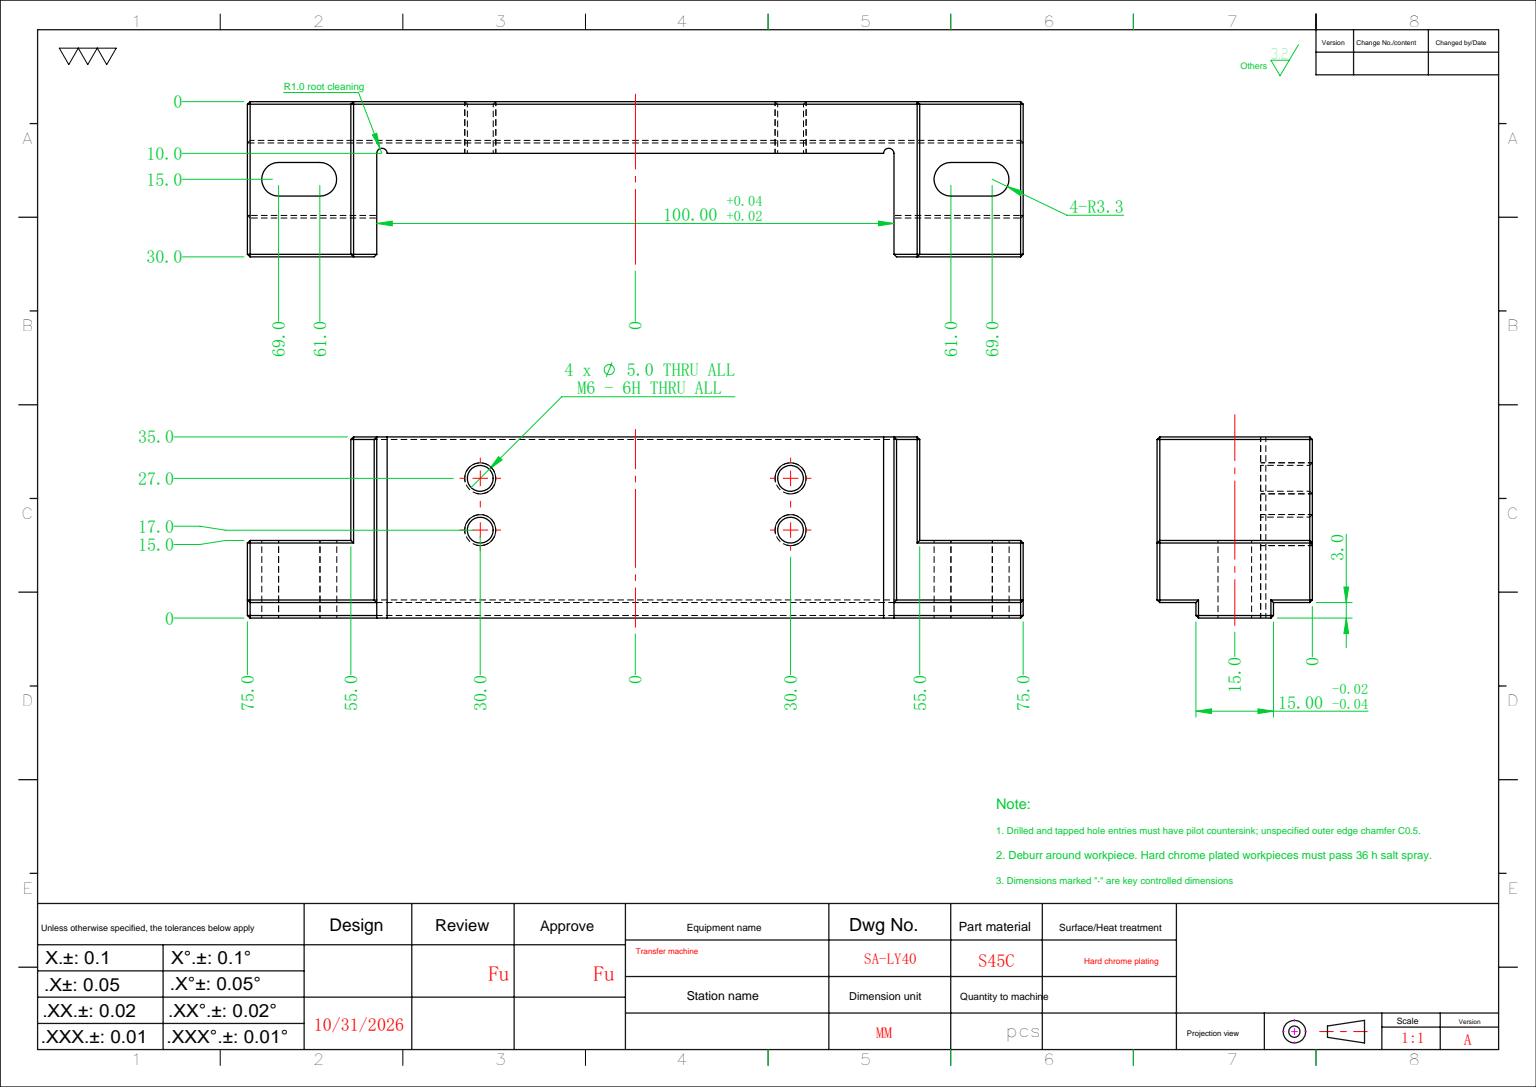
SolidWorks part; units mm, degrees
material "S45C"
ref_plane "前视基准面" through (0, 0, 0) normal (0, 0, 1) x (1, 0, 0)
ref_plane "上视基准面" through (0, 0, 0) normal (0, 1, 0) x (1, 0, 0)
ref_plane "右视基准面" through (0, 0, 0) normal (1, 0, 0) x (0, 0, -1)
sketch "草图1" plane through (0, 0, 0) normal (0, 0, 1) x (1, 0, 0)
  line L0 (0, 0) -> (116.7587, 0) construction
  line L1 (0, 0) -> (0, 69.0405) construction
  line L2 (-75, 0) -> (-75, 15)
  line L3 (-75, 15) -> (-55, 15)
  line L4 (-55, 15) -> (-55, 35)
  line L5 (55, 15) -> (55, 35)
  line L6 (75, 15) -> (55, 15)
  line L7 (75, 0) -> (75, 15)
  line L8 (-75, 0) -> (75, 0)
  line L9 (-55, 35) -> (55, 35)
  dimension "D1" = 150
  dimension "D2" = 110
  dimension "D3" = 15
  dimension "D4" = 35
extrude "凸台-拉伸1" add sketch "草图1" along normal mid plane 30
sketch "草图2" plane through (-75, 0, 0) normal (-1, 0, 0) x (0, 0, 1)
  line L0 (0, 0) -> (0, 17.2771) construction
  line L1 (-15, 0) -> (-7.5, 0)
  line L2 (-15, 0) -> (-15, 3)
  line L3 (-15, 3) -> (-7.5, 3)
  line L4 (-7.5, 0) -> (-7.5, 3)
  line L5 (7.5, 0) -> (7.5, 3)
  line L6 (15, 3) -> (7.5, 3)
  line L7 (15, 0) -> (15, 3)
  line L8 (15, 0) -> (7.5, 0)
  dimension "D1" = 15
  dimension "D2" = 3
extrude "切除-拉伸1" cut sketch "草图2" against normal through all
sketch "草图3" plane through (0, 35, 0) normal (0, 1, 0) x (1, 0, 0)
  line L0 (55, -15) -> (-55, -15) construction
  line L1 (-50, -15) -> (50, -15)
  line L2 (-50, -15) -> (-50, 5)
  line L3 (-50, 5) -> (50, 5)
  line L4 (50, -15) -> (50, 5)
  line L5 (0, 0) -> (0, -41.4975) construction
  dimension "D1" = 100
  dimension "D2" = 20
extrude "切除-拉伸2" cut sketch "草图3" against normal through all
sketch "草图4" plane through (0, 15, 0) normal (0, 1, 0) x (1, 0, 0)
  line L0 (0, 0) -> (126.1164, 0) construction
  line L1 (0, 0) -> (0, 50.8796) construction
  line L2 (61, 0) -> (69, 0) construction
  line L3 (61, 3.25) -> (69, 3.25)
  line L4 (61, -3.25) -> (69, -3.25)
  line L5 (-61, 0) -> (-69, 0) construction
  line L6 (-61, 3.25) -> (-69, 3.25)
  line L7 (-61, -3.25) -> (-69, -3.25)
  arc A0 (61, 3.25) -> (61, -3.25) centre (61, 0) ccw
  arc A1 (69, -3.25) -> (69, 3.25) centre (69, 0) ccw
  arc A2 (-61, 3.25) -> (-61, -3.25) centre (-61, 0) cw
  arc A3 (-69, -3.25) -> (-69, 3.25) centre (-69, 0) cw
  point P6 (65, 0)
  point P13 (-65, 0)
  dimension "D2" = 6.5
  dimension "D1" = 130
  dimension "D3" = 8
extrude "切除-拉伸3" cut sketch "草图4" against normal blind 30
hole_wizard "M6 螺纹孔1" positions "草图5" profile "草图6" tap size "M6" standard "ISO" end condition through all
sketch "草图5" plane through (0, 0, -5) normal (0, 0, 1) x (1, 0, 0)
  line L0 (0, 0) -> (0, 47.6129) construction
  line L2 (-50, 0) -> (50, 0) construction
  point P0 (-30, 17)
  point P11 (30, 17)
  dimension "D2" = 60
  dimension "D3" = 17
sketch "草图6" plane through (-30, 17, -5) normal (1, 0, 0) x (0, -1, 0)
  line L0 (0, 0) -> (0, 10)
  line L1 (0, 10) -> (2.5, 10)
  line L2 (2.5, 10) -> (2.5, 0)
  line L5 (2.5, 0) -> (0, 0)
  line L11 (0, -6.35) -> (0, 107.95) construction
  dimension "通孔螺纹孔钻头直径" = 5
  dimension "通孔螺纹孔钻头深度" = 10
cosmetic thread "孔螺蚊线1" parameters "D1"=12, "D2"=6
cosmetic thread "孔螺蚊线2" parameters "D1"=12, "D2"=6
pattern_linear "阵列(线性)1" count 2 spacing 10 along (0, 1, 0) of "M6 螺纹孔1"
chamfer "倒角1" distance 0.5 angle 45 41 edges at (32.5, 17, -15) (-27.5, 17, -15) (32.5, 27, -15) (-27.5, 27, -15) (65, 15, -15) (55, 25, -15) (0, 35, -15) (-55, 25, -15) (-65, 15, -15) (0, 3, -15) (75, 0, 0) (62.5, 0, 7.5) (75, 1.5, 7.5) (75, 3, 11.25) (-62.5, 3, 15) (-50, 19, 15) (-52.5, 35, 15) (-55, 35, 0) (-55, 25, 15) (-65, 15, 15) (-75, 15, 0) (-75, 9, 15) (-75, 3, 11.25) (-75, 1.5, 7.5) (-62.5, 0, 7.5) (-75, 0, 0) (-75, 9, -15) (-75, 3, -11.25) (-75, 1.5, -7.5) (0, 0, -7.5) (75, 1.5, -7.5) (75, 3, -11.25) (75, 9, -15) (75, 15, 0) (52.5, 35, 15) (50, 19, 15) (62.5, 3, 15) (75, 9, 15) (65, 15, 15) (55, 25, 15) (55, 35, 0)
sketch "草图7" plane through (0, 35, 0) normal (0, 1, 0) x (1, 0, 0)
  line L0 (50, 5) -> (-50, 5) construction
  circle A0 centre (-49, 5) radius 1
  circle A1 centre (49, 5) radius 1
  dimension "D1" = 2
extrude "切除-拉伸4" cut sketch "草图7" against normal through all
